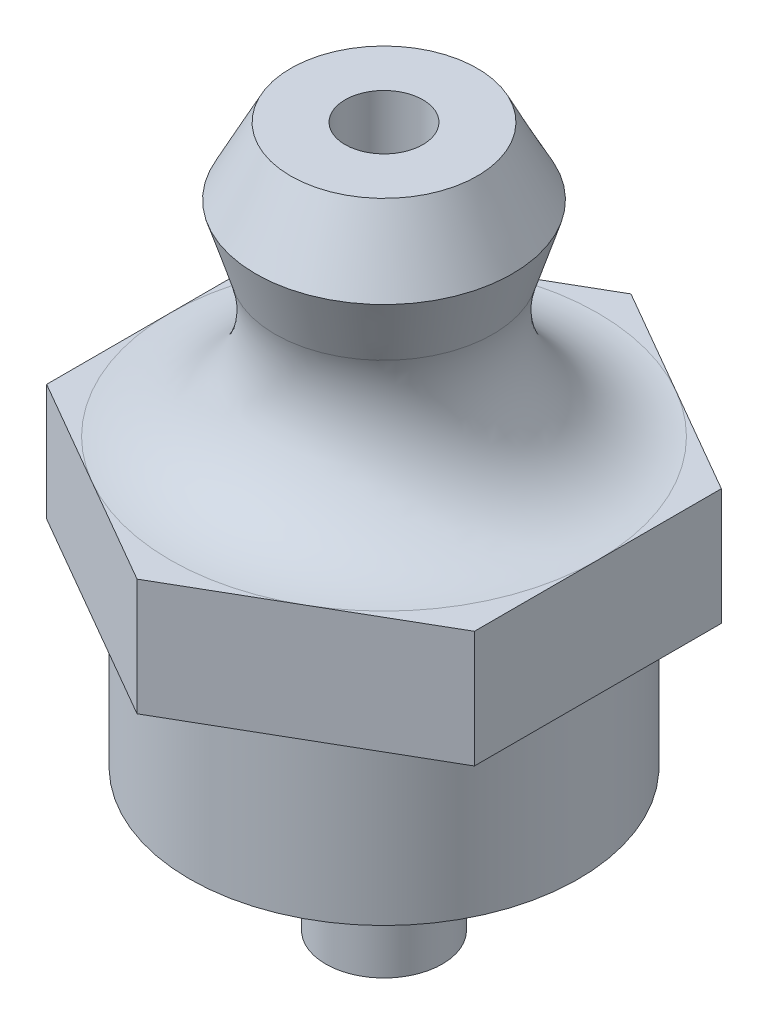
SolidWorks part; units mm, degrees
ref_plane "前视基准面" through (0, 0, 0) normal (0, 0, 1) x (1, 0, 0)
ref_plane "上视基准面" through (0, 0, 0) normal (0, 1, 0) x (1, 0, 0)
ref_plane "右视基准面" through (0, 0, 0) normal (1, 0, 0) x (0, 0, -1)
sketch "草图1" plane through (0, 0, 0) normal (0, 0, 1) x (1, 0, 0)
  line L0 (-1, 18) -> (-2.4, 18)
  line L1 (0, 0) -> (0, -3.114) construction
  line L2 (-2.4, 18) -> (-3.3, 16.2711)
  line L3 (-3.3, 16.2711) -> (-2.8, 14.6756)
  line L4 (0, 11) -> (-6.7881, 11) construction
  line L5 (0, 8) -> (-2.9677, 8) construction
  line L6 (-1, 0) -> (-1.5, 0)
  line L7 (-1.5, 0) -> (-1.5, 1.822)
  line L8 (-1.5, 1.822) -> (-5, 3.644)
  line L9 (-5, 3.644) -> (-5, 8)
  line L10 (-5, 8) -> (-5.5, 8)
  line L11 (-5.5, 8) -> (-5.5, 11)
  line L12 (-1, 0) -> (-1, 18)
  line L13 (-5, 3.644) -> (-5, 1.822) construction
  arc A0 (-5.5, 11) -> (-2.8, 14.6756) centre (-5.5, 13.8295) ccw
  dimension "D1" = 6.6
  dimension "hm" = 18
  dimension "d5" = 117.5
  dimension "D2" = 4.8
  dimension "h1" = 7
  dimension "h" = 10
  dimension "d" = 10
  dimension "sm" = 11
  dimension "D4" = 5.6
  dimension "D6" = 117.5
  dimension "D7" = 3
  dimension "D8" = 2
revolve "旋转2" add sketch "草图1" angle 360 about L1
sketch "草图2" plane through (0, 8, 0) normal (0, -1, 0) x (1, 0, 0)
  line L1 (-5.5, 3.1754) -> (-5.5, -3.1754)
  line L2 (-5.5, -3.1754) -> (0, -6.3509)
  line L3 (0, -6.3509) -> (5.5, -3.1754)
  line L4 (5.5, -3.1754) -> (5.5, 3.1754)
  line L5 (5.5, 3.1754) -> (0, 6.3509)
  line L6 (0, 6.3509) -> (-5.5, 3.1754)
  circle A0 centre (0, 0) radius 5.5 construction
  circle A1 centre (0, 0) radius 5.5 construction
extrude "拉伸1" add sketch "草图2" against normal up to vertex (3 mm away) up to point (-5.5, 11, 0)
